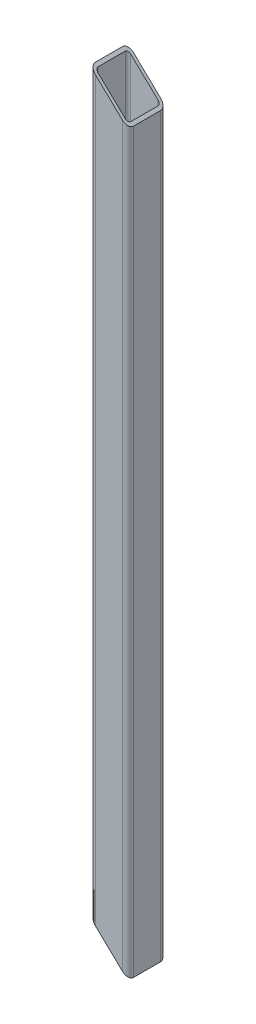
SolidWorks part; units mm, degrees
material "Q235B"
ref_plane "Front Plane" through (0, 0, 0) normal (0, 0, 1) x (1, 0, 0)
ref_plane "Top Plane" through (0, 0, 0) normal (0, 1, 0) x (1, 0, 0)
ref_plane "Right Plane" through (0, 0, 0) normal (1, 0, 0) x (0, 0, -1)
sketch "18 (ProfileFeature) (+7 more in 7 files) Sketch1" plane through (0, 0, 0) normal (0, 0, 1) x (1, 0, 0)
  line L0 (0, 0) -> (0, 1420.5)
  dimension "D1" = 1420.5
other "19 (WeldMemberFeat) (+4 more in 5 files) Cold-formed hollow square steel (GB/T 6728-2002) 70×70×5(1)"
ref_plane "Plane1" through (0, 0, 0) normal (0, 1, 0) x (-1, 0, 0)
sketch "Sketch1" plane through (0, 0, 0) normal (0, 1, 0) x (-1, 0, 0)
  line L0 (-25, -30) -> (25, -30)
  line L1 (-30, -25) -> (-30, 25)
  line L2 (25, 30) -> (-25, 30)
  line L3 (30, 25) -> (30, -25)
  line L4 (-25, -35) -> (25, -35)
  line L5 (-35, -25) -> (-35, 25)
  line L6 (25, 35) -> (-25, 35)
  line L7 (35, 25) -> (35, -25)
  arc A0 (35, 25) -> (25, 35) centre (25, 25) ccw
  arc A1 (25, -35) -> (35, -25) centre (25, -25) ccw
  arc A2 (-35, -25) -> (-25, -35) centre (-25, -25) ccw
  arc A3 (-25, 35) -> (-35, 25) centre (-25, 25) ccw
  arc A4 (-25, 30) -> (-30, 25) centre (-25, 25) ccw
  arc A5 (30, 25) -> (25, 30) centre (25, 25) ccw
  arc A6 (25, -30) -> (30, -25) centre (25, -25) ccw
  arc A7 (-30, -25) -> (-25, -30) centre (-25, -25) ccw
  point P0 (-35, 0)
  point P1 (35, 0)
  point P2 (0, 35)
  point P3 (0, -35)
  point P4 (0, 0)
  point P5 (-35, -35)
  point P6 (35, -35)
  point P7 (35, 35)
  point P8 (-35, 35)
  point P33 (0, 0)
  dimension "D1" = 10
  dimension "D2" = 70
  dimension "D3" = 5
sketch "Sketch2" plane through (0, 0, 35) normal (0, 0, 1) x (1, 0, 0)
  line L1 (-35, 1420.5) -> (-35, 0) construction
  line L4 (-35, 66.7136) -> (35, 0)
  line L5 (35, 0) -> (-35, 0)
  line L6 (-35, 0) -> (-35, 66.7136)
  line L7 (-35, 1420.5) -> (35, 1353.7864)
  line L8 (35, 1420.5) -> (35, 0) construction
  line L9 (35, 1353.7864) -> (35, 1420.5)
  line L10 (35, 1420.5) -> (-35, 1420.5)
  dimension "D1" = 980
extrude "Cut-Extrude1" cut sketch "Sketch2" against normal through all both and the other way through all
